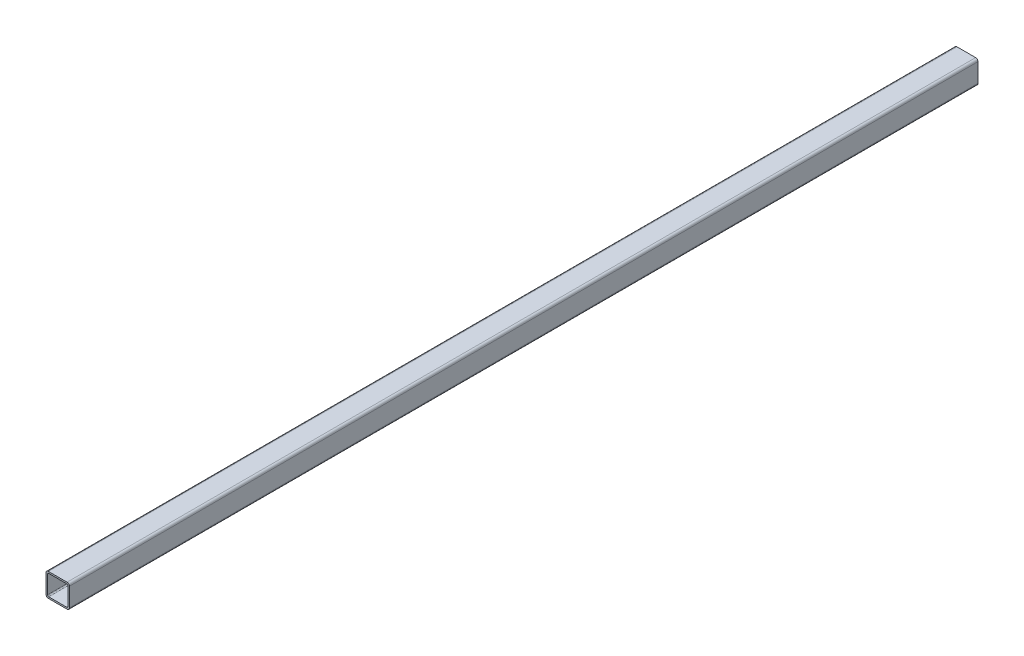
SolidWorks part; units mm, degrees
material "Q235"
ref_plane "Front Plane" through (0, 0, 0) normal (0, 0, 1) x (1, 0, 0)
ref_plane "Top Plane" through (0, 0, 0) normal (0, 1, 0) x (1, 0, 0)
ref_plane "Right Plane" through (0, 0, 0) normal (1, 0, 0) x (0, 0, -1)
sketch "Sketch1" plane through (0, 0, 0) normal (0, 0, 1) x (1, 0, 0)
  line L1 (-30, -30) -> (30, -30)
  line L2 (-30, -30) -> (-30, 30)
  line L3 (-30, 30) -> (30, 30)
  line L4 (30, -30) -> (30, 30)
  line L5 (-30, -30) -> (30, 30) construction
  line L6 (-30, 30) -> (30, -30) construction
  line L7 (-26, -26) -> (26, -26)
  line L8 (-26, -26) -> (-26, 26)
  line L9 (-26, 26) -> (26, 26)
  line L10 (26, -26) -> (26, 26)
  line L11 (-26, -26) -> (26, 26) construction
  line L12 (-26, 26) -> (26, -26) construction
  point P0 (0, 0)
  point P5 (0, 0)
  dimension "D1" = 4
  dimension "D2" = 60
  dimension "D3" = 60
extrude "Boss-Extrude1" add sketch "Sketch1" along normal mid plane 2330
fillet "Fillet1" radius 6 4 edges at (30, -30, 0) (-30, -30, 0) (30, 30, 0) (-30, 30, 0)
fillet "Fillet2" radius 3 4 edges at (26, -26, 0) (-26, -26, 0) (26, 26, 0) (-26, 26, 0)
